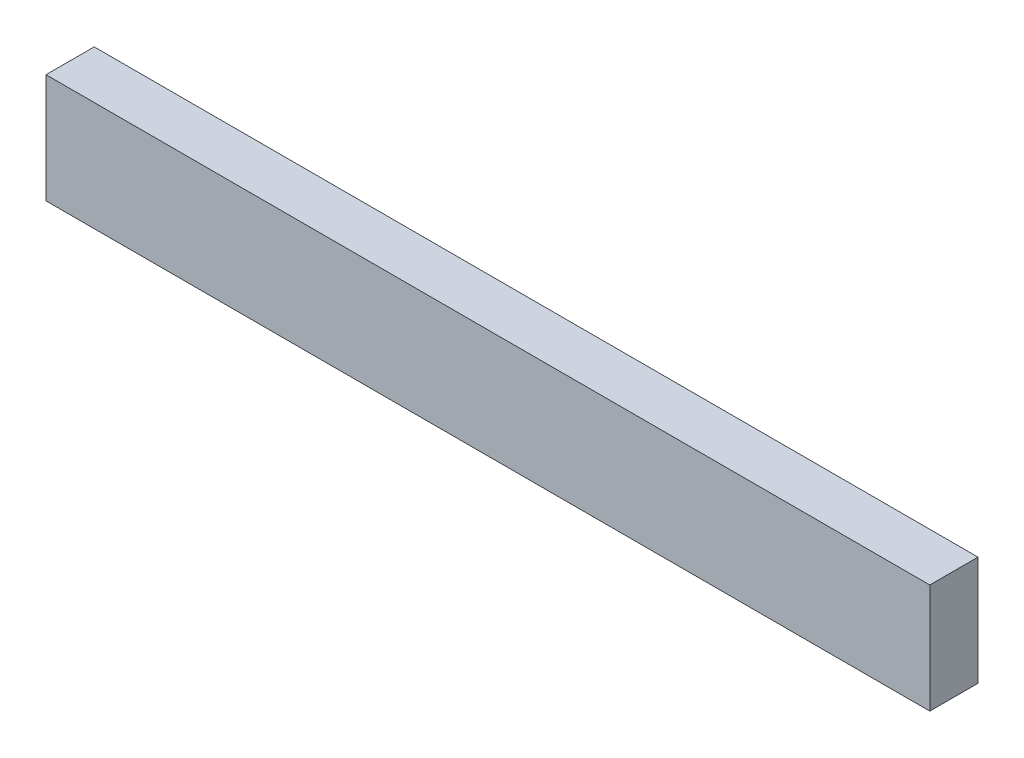
from build123d import *

# Parameters (mm, degrees)
SKETCH_1_W      = 275
SKETCH_1_H      = 34
EXTRUDE_1_DEPTH = 15


with BuildPart() as part:
    # 草图1 → 凸台-拉伸1 (new body)
    with BuildSketch(Plane.XY):
        Rectangle(SKETCH_1_W, SKETCH_1_H)
    extrude(amount=EXTRUDE_1_DEPTH)


solid = part.part
